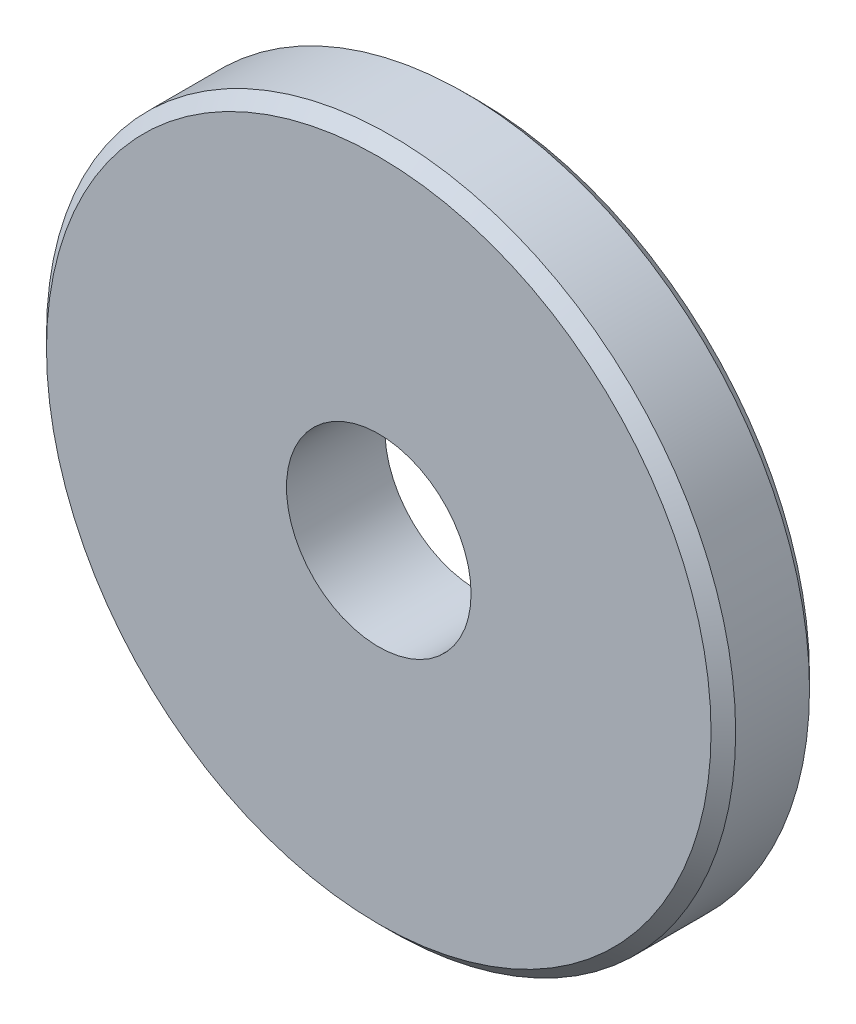
SolidWorks part; units mm, degrees
ref_plane "前视基准面" through (0, 0, 0) normal (0, 0, 1) x (1, 0, 0)
ref_plane "上视基准面" through (0, 0, 0) normal (0, 1, 0) x (1, 0, 0)
ref_plane "右视基准面" through (0, 0, 0) normal (1, 0, 0) x (0, 0, -1)
sketch "草图1" plane through (0, 0, 0) normal (0, 0, 1) x (1, 0, 0)
  circle A0 centre (0, 0) radius 28
  circle A1 centre (0, 0) radius 7.5
  dimension "D1" = 56
  dimension "D2" = 15
extrude "凸台-拉伸1" add sketch "草图1" along normal blind 8
chamfer "倒角1" distance 1 angle 45 2 edges at (28, 0, 0) (28, 0, 8)
